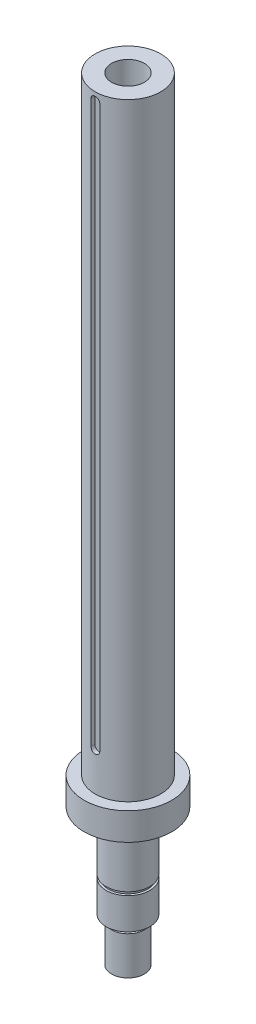
from build123d import *

# Parameters (mm, degrees)
SKETCH_2_R          = 15
CUT_EXTRUDE_1_DEPTH = 50
CUT_EXTRUDE_START   = -7.5
SKETCH_3_W          = 8
SKETCH_3_H          = 7
CUT_EXTRUDE_2_DEPTH = 512.59
CUT_EXTRUDE_3_DEPTH = 7


with BuildPart() as part:
    # 草图1 → 旋转1 (revolve)
    with BuildSketch(Plane.XY, mode=Mode.PRIVATE) as revolve_1_sk:
        Polygon((0, -243.614201173), (15, -243.614201173), (15, -208.614201173), (10, -208.614201173), (10, -203.614201173), (20, -203.614201173), (20, -174.914201173), (18, -174.914201173), (18, -171.914201173), (20, -171.914201173), (20, -118.614201173), (40, -118.614201173), (40, -93.614201173), (30, -93.614201173), (30, 461.975798827), (0, 461.975798827), align=None)
    revolve(revolve_1_sk.sketch.rotate(Axis((0, 247.860200322, 0), (0, -1, 0)), 90), axis=Axis((0, 247.860200322, 0), (0, -1, 0)))

    # 草图2 → 切除-拉伸1 (cut)
    with BuildSketch(Plane(origin=(0, 461.975798827, 0), x_dir=(1, 0, 0), z_dir=(0, 1, 0))):
        with Locations(Location((0, 0, 0), (0, 0, 270))):
            Circle(SKETCH_2_R)
    extrude(amount=-CUT_EXTRUDE_1_DEPTH, mode=Mode.SUBTRACT)

    # 草图3 → 切除-拉伸2 (cut)
    with BuildSketch(Plane(origin=(0, 461.975798827, 0), x_dir=(1, 0, 0), z_dir=(0, 1, 0)).offset(CUT_EXTRUDE_START)):
        with Locations((0, -29.732137495)):
            Rectangle(SKETCH_3_W, SKETCH_3_H)
    extrude(amount=-CUT_EXTRUDE_2_DEPTH, mode=Mode.SUBTRACT)

    # 草图4 → 切除-拉伸3 (cut)
    with BuildSketch(Plane.XY.offset(26.232137495)):
        with BuildLine():
            Line((4, -58.114201173), (-4, -58.114201173))
            ThreePointArc((-4, -58.114201173), (0, -62.114201173), (4, -58.114201173))
        make_face()
        with BuildLine():
            Line((-4, 454.475798827), (4, 454.475798827))
            ThreePointArc((4, 454.475798827), (0, 458.475798827), (-4, 454.475798827))
        make_face()
    extrude(amount=CUT_EXTRUDE_3_DEPTH, mode=Mode.SUBTRACT)


solid = part.part
